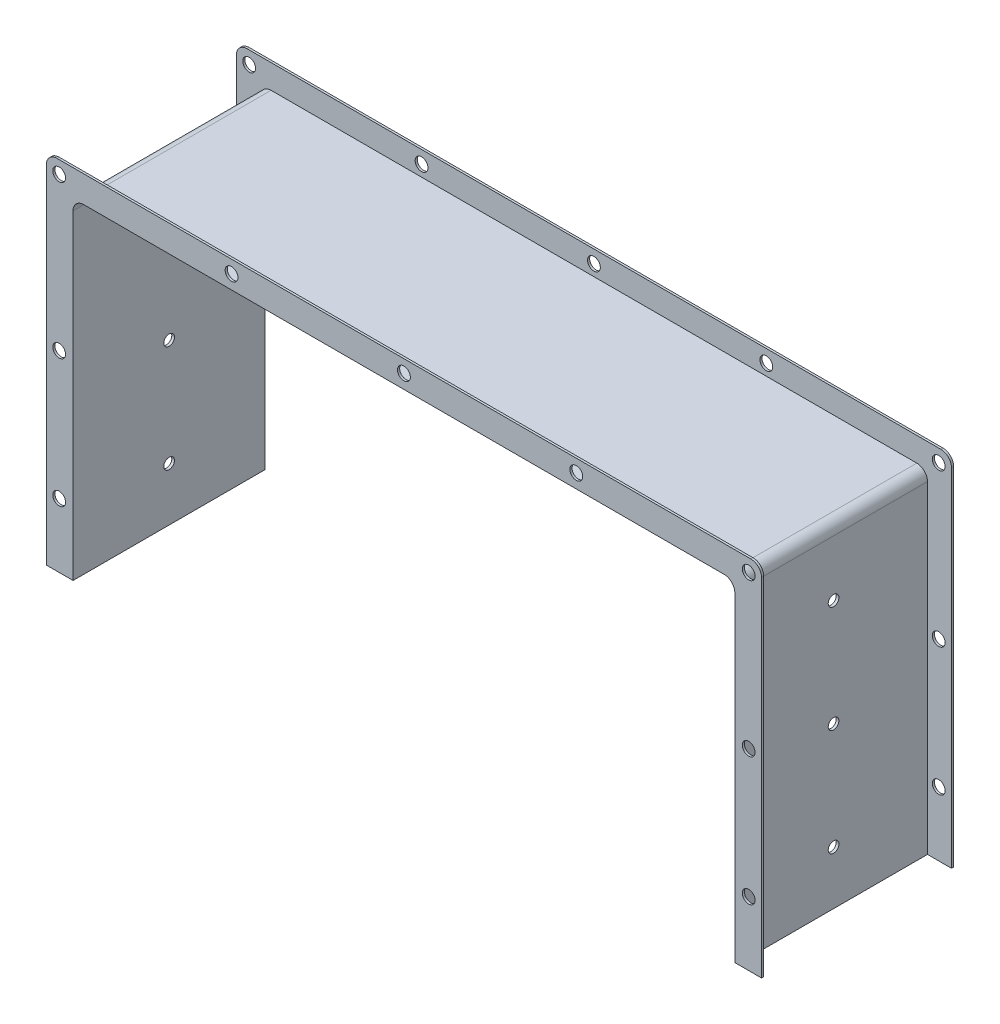
SolidWorks part; units mm, degrees
ref_plane "Front Plane" through (0, 0, 0) normal (0, 0, 1) x (1, 0, 0)
ref_plane "Top Plane" through (0, 0, 0) normal (0, 1, 0) x (1, 0, 0)
ref_plane "Right Plane" through (0, 0, 0) normal (1, 0, 0) x (0, 0, -1)
sketch "Sketch1" plane through (0, 0, 0) normal (0, 0, 1) x (1, 0, 0)
  line L0 (0, 0) -> (0, -323.5607) construction
  line L2 (-335, -167.5) -> (-335, 157.5)
  line L3 (-325, 167.5) -> (325, 167.5)
  line L4 (335, -167.5) -> (335, 157.5)
  line L5 (-335, -167.5) -> (335, 167.5) construction
  line L6 (-335, 167.5) -> (335, -167.5) construction
  line L7 (-310, -167.5) -> (-310, 132.5)
  line L8 (-300, 142.5) -> (300, 142.5)
  line L9 (310, 132.5) -> (310, -167.5)
  line L10 (-335, -167.5) -> (-310, -167.5)
  line L11 (310, -167.5) -> (335, -167.5)
  arc A0 (325, 167.5) -> (335, 157.5) centre (325, 157.5) cw
  arc A1 (-335, 157.5) -> (-325, 167.5) centre (-325, 157.5) cw
  arc A2 (310, 132.5) -> (300, 142.5) centre (300, 132.5) ccw
  arc A3 (-310, 132.5) -> (-300, 142.5) centre (-300, 132.5) cw
  point P0 (0, 0)
  dimension "D3" = 10
  dimension "D7" = 10
  dimension "D1" = 670
  dimension "D2" = 335
  dimension "D4" = 25
  dimension "D5" = 25
  dimension "D6" = 25
extrude "Boss-Extrude1" add sketch "Sketch1" along normal blind 2
sketch "Sketch2" plane through (0, 0, 0) normal (0, 0, -1) x (-1, 0, 0)
  line L0 (310, -167.5) -> (310, 132.5) construction
  line L1 (300, 142.5) -> (-300, 142.5) construction
  line L2 (-310, 132.5) -> (-310, -167.5) construction
  line L3 (310, -167.5) -> (310, 132.5)
  line L4 (300, 142.5) -> (-300, 142.5)
  line L5 (-310, 132.5) -> (-310, -167.5)
  line L6 (-310, -167.5) -> (-312.5, -167.5)
  line L8 (-310, -167.5) -> (-335, -167.5) construction
  line L9 (-312.5, -167.5) -> (-312.5, 135)
  line L10 (-302.5, 145) -> (302.5, 145)
  line L11 (312.5, 135) -> (312.5, -167.5)
  line L12 (335, -167.5) -> (310, -167.5) construction
  line L13 (312.5, -167.5) -> (310, -167.5)
  arc A0 (310, 132.5) -> (300, 142.5) centre (300, 132.5) ccw construction
  arc A1 (-300, 142.5) -> (-310, 132.5) centre (-300, 132.5) ccw construction
  arc A2 (310, 132.5) -> (300, 142.5) centre (300, 132.5) ccw
  arc A3 (-300, 142.5) -> (-310, 132.5) centre (-300, 132.5) ccw
  arc A4 (312.5, 135) -> (302.5, 145) centre (302.5, 135) ccw
  arc A5 (-312.5, 135) -> (-302.5, 145) centre (-302.5, 135) cw
  dimension "D4" = 10
  dimension "D1" = 2.5
  dimension "D2" = 2.5
  dimension "D3" = 2.5
extrude "Boss-Extrude2" add sketch "Sketch2" along normal blind 178
sketch "Sketch3" plane through (0, 0, 0) normal (0, 0, -1) x (-1, 0, 0)
  line L0 (-325, 167.5) -> (325, 167.5) construction
  line L1 (0, 0) -> (0, -133.1296) construction
  line L2 (-335, -167.5) -> (-335, 157.5) construction
  line L3 (-312.5, -167.5) -> (-335, -167.5) construction
  circle A0 centre (0, 155.5) radius 6
  circle A1 centre (-161.5, 155.5) radius 6
  circle A2 centre (-323, 12.5) radius 6
  circle A3 centre (-323, -107.5) radius 6
  circle A4 centre (-323, 155.5) radius 6
  circle A5 centre (323, 155.5) radius 6
  circle A6 centre (323, -107.5) radius 6
  circle A7 centre (323, 12.5) radius 6
  circle A8 centre (161.5, 155.5) radius 6
  dimension "D1" = 12
  dimension "D3" = 12
  dimension "D4" = 60
  dimension "D2" = 12
  dimension "D5" = 120
  dimension "D6" = 161.5
extrude "Cut-Extrude1" cut sketch "Sketch3" against normal through all and the other way through all
sketch "Sketch4" plane through (312.5, 0, 0) normal (1, 0, 0) x (0, 0, -1)
  line L0 (-2, -167.5) -> (-2, 157.5) construction
  line L1 (-2, 167.5) -> (0, 167.5) construction
  circle A0 centre (88, 82.5) radius 5
  circle A1 centre (88, -17.5) radius 5
  circle A2 centre (88, -117.5) radius 5
  dimension "D1" = 90
  dimension "D3" = 10
  dimension "D4" = 100
  dimension "D2" = 85
  dimension "D5" = 100
extrude "Cut-Extrude2" cut sketch "Sketch4" against normal through all
sketch "Sketch5" plane through (0, 0, -178) normal (0, 0, -1) x (-1, 0, 0)
  line L8 (-312.5, -167.5) -> (-312.5, 135)
  line L9 (-302.5, 145) -> (302.5, 145)
  line L10 (312.5, 135) -> (312.5, -167.5)
  line L11 (312.5, -167.5) -> (335, -167.5)
  line L12 (335, -167.5) -> (335, 157.5)
  line L13 (325, 167.5) -> (-325, 167.5)
  line L14 (-335, 157.5) -> (-335, -167.5)
  line L15 (-335, -167.5) -> (-312.5, -167.5)
  line L16 (-312.5, -167.5) -> (-312.5, 135)
  line L17 (-302.5, 145) -> (302.5, 145)
  line L18 (312.5, 135) -> (312.5, -167.5)
  line L19 (312.5, -167.5) -> (335, -167.5)
  line L20 (335, -167.5) -> (335, 157.5)
  line L21 (325, 167.5) -> (-325, 167.5)
  line L22 (-335, 157.5) -> (-335, -167.5)
  line L23 (-335, -167.5) -> (-312.5, -167.5)
  circle A1 centre (-323, -107.5) radius 6
  circle A2 centre (-323, -107.5) radius 6
  circle A3 centre (-323, 12.5) radius 6
  arc A4 (-302.5, 145) -> (-312.5, 135) centre (-302.5, 135) ccw
  arc A5 (312.5, 135) -> (302.5, 145) centre (302.5, 135) ccw
  arc A6 (335, 157.5) -> (325, 167.5) centre (325, 157.5) ccw
  arc A7 (-325, 167.5) -> (-335, 157.5) centre (-325, 157.5) ccw
  arc A8 (-302.5, 145) -> (-312.5, 135) centre (-302.5, 135) ccw
  arc A9 (312.5, 135) -> (302.5, 145) centre (302.5, 135) ccw
  arc A10 (335, 157.5) -> (325, 167.5) centre (325, 157.5) ccw
  arc A11 (-325, 167.5) -> (-335, 157.5) centre (-325, 157.5) ccw
  circle A12 centre (-323, 12.5) radius 6
  circle A13 centre (-161.5, 155.5) radius 6
  circle A14 centre (-161.5, 155.5) radius 6
  circle A15 centre (0, 155.5) radius 6
  circle A16 centre (0, 155.5) radius 6
  circle A17 centre (161.5, 155.5) radius 6
  circle A18 centre (161.5, 155.5) radius 6
  circle A19 centre (323, 12.5) radius 6
  circle A20 centre (323, 12.5) radius 6
  circle A21 centre (323, -107.5) radius 6
  circle A22 centre (323, -107.5) radius 6
  circle A23 centre (323, 155.5) radius 6
  circle A24 centre (323, 155.5) radius 6
  circle A25 centre (-323, 155.5) radius 6
  circle A26 centre (-323, 155.5) radius 6
  dimension "D1" = 0
  dimension "D2" = 0
  dimension "D3" = 0
  dimension "D4" = 0
  dimension "D5" = 0
  dimension "D6" = 0
  dimension "D7" = 0
  dimension "D8" = 0
  dimension "D9" = 0
  dimension "D10" = 0
extrude "Boss-Extrude3" add sketch "Sketch5" against normal blind 2
